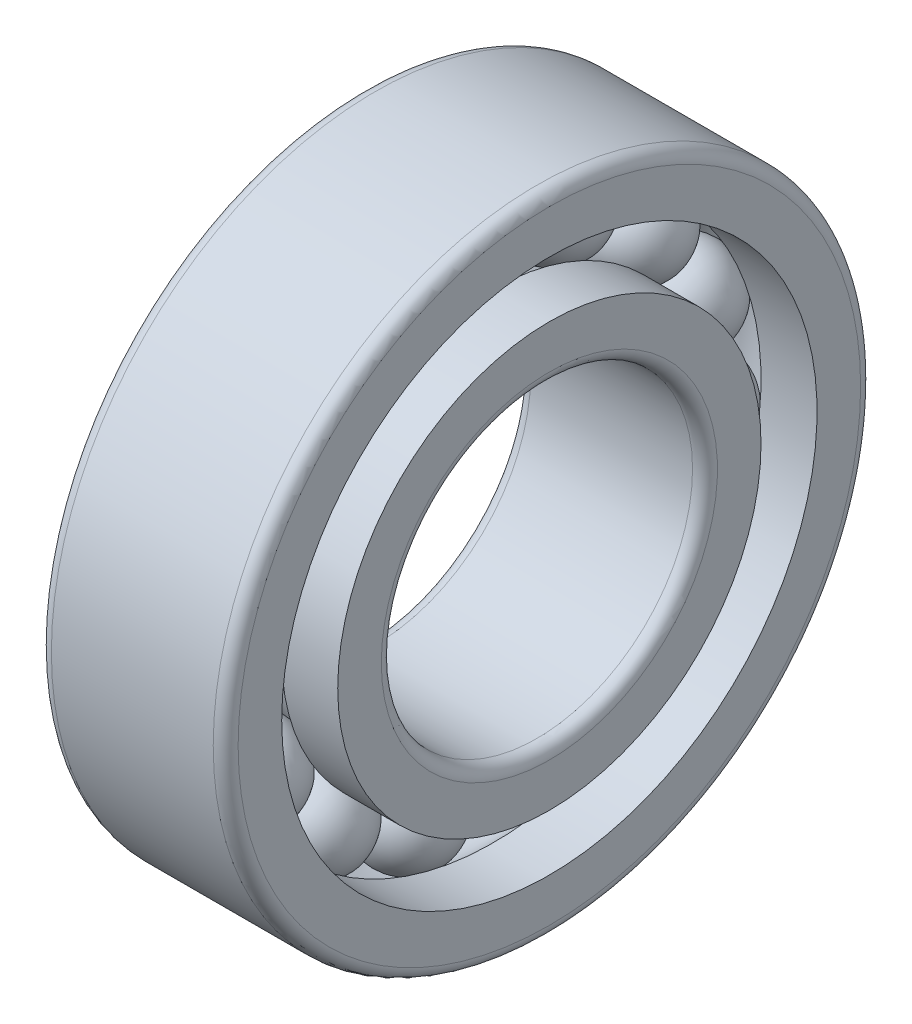
from build123d import *

# Parameters (mm, degrees)
CIRPATTERN5_COUNT = 15


with BuildPart() as part:
    # Sketch2 → Revolve1 (revolve)
    with BuildSketch(Plane.XY, mode=Mode.PRIVATE) as revolve1_sk:
        with BuildLine():
            Line((-7, 17), (-7.5, 17))
            Line((-7.5, 17), (-7.5, 16))
            Line((-7.5, 16), (-7.5, 13.5))
            ThreePointArc((-7.5, 13.5), (-7.207106781, 12.792893219), (-6.5, 12.5))
            Line((-6.5, 12.5), (6.5, 12.5))
            ThreePointArc((6.5, 12.5), (7.207106781, 12.792893219), (7.5, 13.5))
            Line((7.5, 13.5), (7.5, 16))
            Line((7.5, 16), (7.5, 17))
            Line((7.5, 17), (6.5, 17))
            Line((6.5, 17), (3, 17))
            ThreePointArc((3, 17), (0, 15.5), (-3, 17))
            Line((-3, 17), (-5, 17))
            Line((-5, 17), (-5, 16))
            Line((-5, 16), (-6, 16))
            Line((-6, 16), (-7, 17))
        make_face()
        with BuildLine():
            Line((-7.5, 21.5), (-7, 21.5))
            Line((-7, 21.5), (-6, 22.5))
            Line((-6, 22.5), (-5, 22.5))
            Line((-5, 22.5), (-5, 21.5))
            Line((-5, 21.5), (-3, 21.5))
            ThreePointArc((-3, 21.5), (0, 23), (3, 21.5))
            Line((3, 21.5), (7.5, 21.5))
            Line((7.5, 21.5), (7.5, 25))
            ThreePointArc((7.5, 25), (7.207106781, 25.707106781), (6.5, 26))
            Line((6.5, 26), (-6.5, 26))
            ThreePointArc((-6.5, 26), (-7.207106781, 25.707106781), (-7.5, 25))
            Line((-7.5, 25), (-7.5, 21.5))
        make_face()
    revolve(revolve1_sk.sketch.rotate(Axis((-3.5, 0, 0), (1, 0, 0)), 90), axis=Axis((-3.5, 0, 0), (1, 0, 0)))


with BuildPart() as body_2:
    # Sketch3 → Revolve2 (revolve)
    with BuildSketch(Plane.XY):
        with BuildLine():
            Line((-3.75, 19.25), (3.75, 19.25))
            ThreePointArc((3.75, 19.25), (0, 23), (-3.75, 19.25))
        make_face()
    revolve(axis=Axis((3.75, 19.25, 0), (1, 0, 0)))


with BuildPart() as body_3:
    # Sketch4 → Revolve3 (revolve)
    with BuildSketch(Plane.XY, mode=Mode.PRIVATE) as revolve3_sk:
        Polygon((-7, 21.5), (-7, 17), (-6, 16), (-5, 16), (-5, 17), (-6, 18), (-6, 20.5), (-5, 21.5), (-5, 22.5), (-6, 22.5), align=None)
    revolve(revolve3_sk.sketch.rotate(Axis((-19.927092192, 0, 0), (1, 0, 0)), 90), axis=Axis((-19.927092192, 0, 0), (1, 0, 0)))


with BuildPart() as cirpattern5_1:
    # CirPattern5: pattern copy
    add(body_2.part.rotate(Axis((0, 0, 0), (1, 0, 0)), 1 * 360 / CIRPATTERN5_COUNT))


with BuildPart() as cirpattern5_2:
    # CirPattern5: pattern copy
    add(body_2.part.rotate(Axis((0, 0, 0), (1, 0, 0)), 2 * 360 / CIRPATTERN5_COUNT))


with BuildPart() as cirpattern5_3:
    # CirPattern5: pattern copy
    add(body_2.part.rotate(Axis((0, 0, 0), (1, 0, 0)), 3 * 360 / CIRPATTERN5_COUNT))


with BuildPart() as cirpattern5_4:
    # CirPattern5: pattern copy
    add(body_2.part.rotate(Axis((0, 0, 0), (1, 0, 0)), 4 * 360 / CIRPATTERN5_COUNT))


with BuildPart() as cirpattern5_5:
    # CirPattern5: pattern copy
    add(body_2.part.rotate(Axis((0, 0, 0), (1, 0, 0)), 5 * 360 / CIRPATTERN5_COUNT))


with BuildPart() as cirpattern5_6:
    # CirPattern5: pattern copy
    add(body_2.part.rotate(Axis((0, 0, 0), (1, 0, 0)), 6 * 360 / CIRPATTERN5_COUNT))


with BuildPart() as cirpattern5_7:
    # CirPattern5: pattern copy
    add(body_2.part.rotate(Axis((0, 0, 0), (1, 0, 0)), 7 * 360 / CIRPATTERN5_COUNT))


with BuildPart() as cirpattern5_8:
    # CirPattern5: pattern copy
    add(body_2.part.rotate(Axis((0, 0, 0), (1, 0, 0)), 8 * 360 / CIRPATTERN5_COUNT))


with BuildPart() as cirpattern5_9:
    # CirPattern5: pattern copy
    add(body_2.part.rotate(Axis((0, 0, 0), (1, 0, 0)), 9 * 360 / CIRPATTERN5_COUNT))


with BuildPart() as cirpattern5_10:
    # CirPattern5: pattern copy
    add(body_2.part.rotate(Axis((0, 0, 0), (1, 0, 0)), 10 * 360 / CIRPATTERN5_COUNT))


with BuildPart() as cirpattern5_11:
    # CirPattern5: pattern copy
    add(body_2.part.rotate(Axis((0, 0, 0), (1, 0, 0)), 11 * 360 / CIRPATTERN5_COUNT))


with BuildPart() as cirpattern5_12:
    # CirPattern5: pattern copy
    add(body_2.part.rotate(Axis((0, 0, 0), (1, 0, 0)), 12 * 360 / CIRPATTERN5_COUNT))


with BuildPart() as cirpattern5_13:
    # CirPattern5: pattern copy
    add(body_2.part.rotate(Axis((0, 0, 0), (1, 0, 0)), 13 * 360 / CIRPATTERN5_COUNT))


with BuildPart() as cirpattern5_14:
    # CirPattern5: pattern copy
    add(body_2.part.rotate(Axis((0, 0, 0), (1, 0, 0)), 14 * 360 / CIRPATTERN5_COUNT))


solid = Compound([part.part, body_2.part, body_3.part, cirpattern5_1.part, cirpattern5_2.part, cirpattern5_3.part, cirpattern5_4.part, cirpattern5_5.part, cirpattern5_6.part, cirpattern5_7.part, cirpattern5_8.part, cirpattern5_9.part, cirpattern5_10.part, cirpattern5_11.part, cirpattern5_12.part, cirpattern5_13.part, cirpattern5_14.part])
